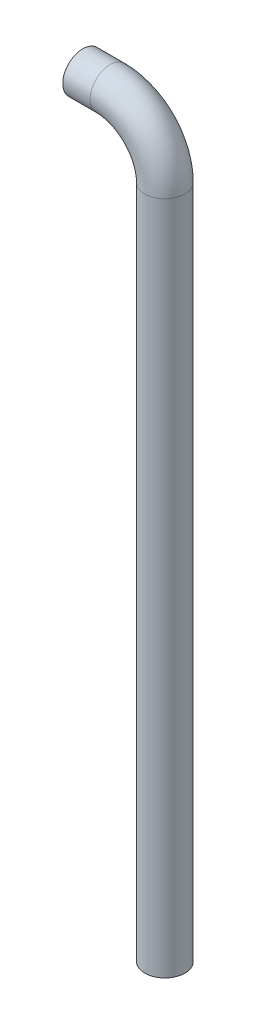
SolidWorks part; units mm, degrees
ref_plane "Front Plane" through (0, 0, 0) normal (0, 0, 1) x (1, 0, 0)
ref_plane "Top Plane" through (0, 0, 0) normal (0, 1, 0) x (1, 0, 0)
ref_plane "Right Plane" through (0, 0, 0) normal (1, 0, 0) x (0, 0, -1)
sketch "Sketch 1" plane through (0, 0, 0) normal (0, 0, 1) x (1, 0, 0)
  line L0 (0, 0) -> (15, 0)
  line L1 (45, -30) -> (45, -400)
  arc A0 (15, 0) -> (45, -30) centre (15, -30) cw
  point P6 (45, 0)
  dimension "D2" = 30
  dimension "D1" = 45
  dimension "D3" = 400
sketch "Sketch 2" plane through (0, 0, 0) normal (1, 0, 0) x (0, 0, -1)
  circle A0 centre (0, 0) radius 11
  circle A1 centre (0, 0) radius 8
  dimension "D1" = 22
  dimension "D2" = 3
sweep "Sweep 1" add profiles "Sketch 2" path "Sketch 1"
